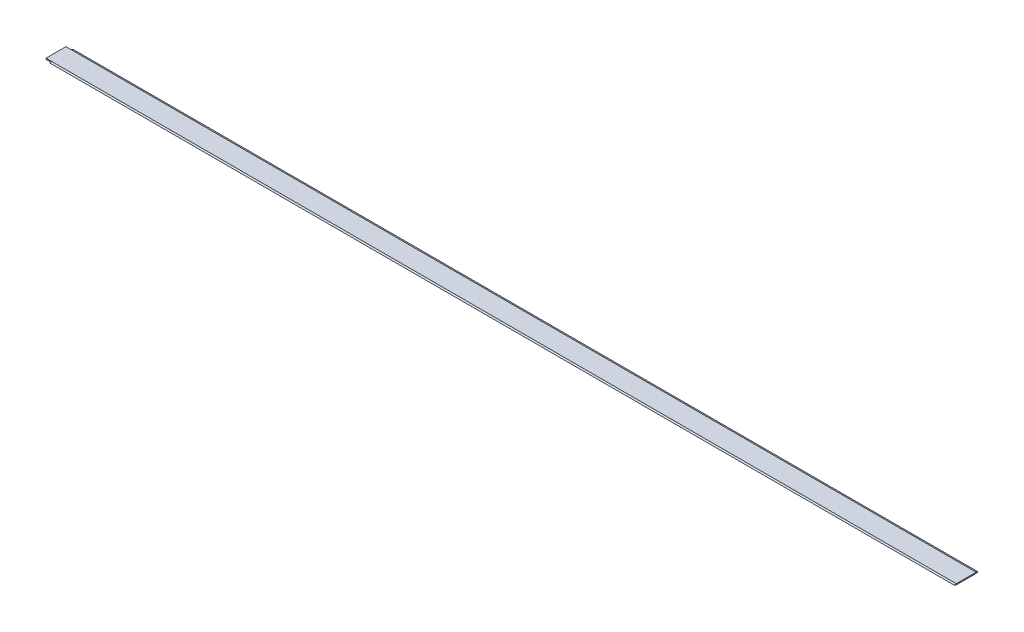
SolidWorks part; units mm, degrees
material "AISI 类型 A2 刀具钢"
ref_plane "Front Plane" through (0, 0, 0) normal (0, 0, 1) x (1, 0, 0)
ref_plane "Top Plane" through (0, 0, 0) normal (0, 1, 0) x (1, 0, 0)
ref_plane "Right Plane" through (0, 0, 0) normal (1, 0, 0) x (0, 0, -1)
other "Configuration Table"
sketch "Sketch1" plane through (0, 0, 0) normal (0, 1, 0) x (1, 0, 0)
  line L1 (-250, -6.5) -> (250, -6.5)
  line L2 (-250, -6.5) -> (-250, 6.5)
  line L3 (-250, 6.5) -> (250, 6.5)
  line L4 (250, -6.5) -> (250, 6.5)
  line L5 (-250, -6.5) -> (250, 6.5) construction
  line L6 (-250, 6.5) -> (250, -6.5) construction
  point P0 (0, 0)
  dimension "D1" = 13
  dimension "D2" = 500
extrude "Boss-Extrude1" add sketch "Sketch1" along normal mid plane 0.6
sketch "Sketch2" plane through (0, 0, 0) normal (1, 0, 0) x (0, 0, -1)
  line L0 (0, 0) -> (0, 1.4628) construction
  line L1 (5.5, 0.3) -> (6.5, 0)
  line L4 (6.5, 0) -> (5.5, -0.3)
  line L6 (5.5, -0.3) -> (7, -0.3)
  line L7 (7, -0.3) -> (7, 0.3)
  line L8 (7, 0.3) -> (5.5, 0.3)
  line L9 (5.5, 0.3) -> (5.5, -0.3) construction
  line L10 (-5.5, 0.3) -> (-5.5, -0.3) construction
  line L11 (-7, 0.3) -> (-5.5, 0.3)
  line L12 (-7, -0.3) -> (-7, 0.3)
  line L13 (-5.5, -0.3) -> (-7, -0.3)
  line L14 (-6.5, 0) -> (-5.5, -0.3)
  line L15 (-5.5, 0.3) -> (-6.5, 0)
  line L16 (6.5, 0.3) -> (6.5, -0.3) construction
  line L17 (-6.5, -0.3) -> (6.5, -0.3) construction
  line L18 (-6.5, 0.3) -> (6.5, 0.3) construction
  dimension "D1" = 1
  dimension "D2" = 1.5
extrude "Cut-Extrude1" cut sketch "Sketch2" against normal through all both and the other way through all
sketch "Sketch3" plane through (-250, 0, 0) normal (-1, 0, 0) x (0, 0, 1)
  line L1 (-5.5, 0.3) -> (5.5, 0.3)
  line L2 (-5.5, 0.3) -> (-5.5, -0.3)
  line L3 (-5.5, -0.3) -> (5.5, -0.3)
  line L4 (5.5, 0.3) -> (5.5, -0.3)
extrude "Boss-Extrude2" add sketch "Sketch3" along normal blind 3
